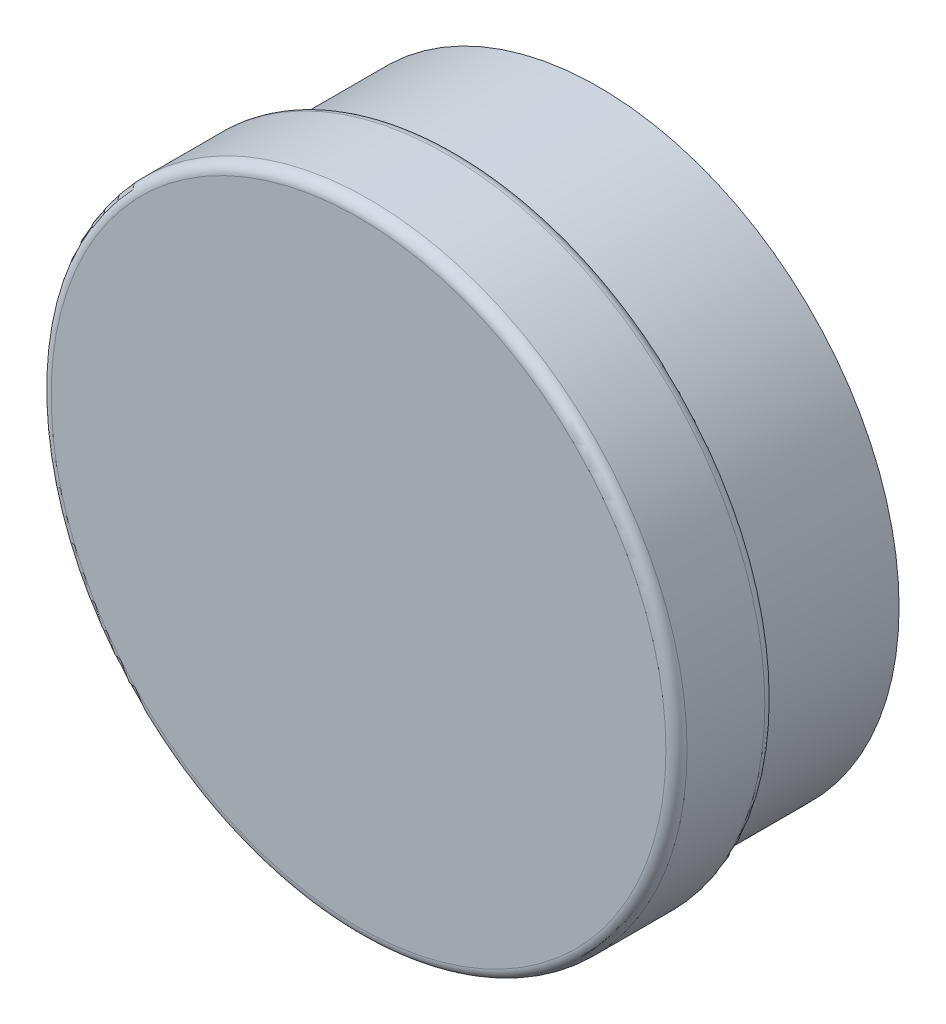
SolidWorks part; units mm, degrees
ref_plane "Front Plane" through (0, 0, 0) normal (0, 0, 1) x (1, 0, 0)
ref_plane "Top Plane" through (0, 0, 0) normal (0, 1, 0) x (1, 0, 0)
ref_plane "Right Plane" through (0, 0, 0) normal (1, 0, 0) x (0, 0, -1)
sketch "Sketch1" plane through (0, 0, 0) normal (0, 0, 1) x (1, 0, 0)
  circle A0 centre (0, 0) radius 8.5
  dimension "D1" = 17
extrude "Boss-Extrude1" add sketch "Sketch1" along normal blind 4
sketch "Sketch2" plane through (0, 0, 4) normal (0, 0, 1) x (1, 0, 0)
  circle A0 centre (0, 0) radius 9
  dimension "D1" = 18
extrude "Boss-Extrude2" add sketch "Sketch2" along normal blind 2.8
fillet "Fillet1" radius 0.3 2 edges at (9, 0, 6.8) (9, 0, 4)
sketch "Sketch3" plane through (0, 0, 0) normal (0, 0, -1) x (-1, 0, 0)
  circle A0 centre (0, 0) radius 1.5
  dimension "D1" = 3
extrude "Cut-Extrude1" cut sketch "Sketch3" against normal blind 5
